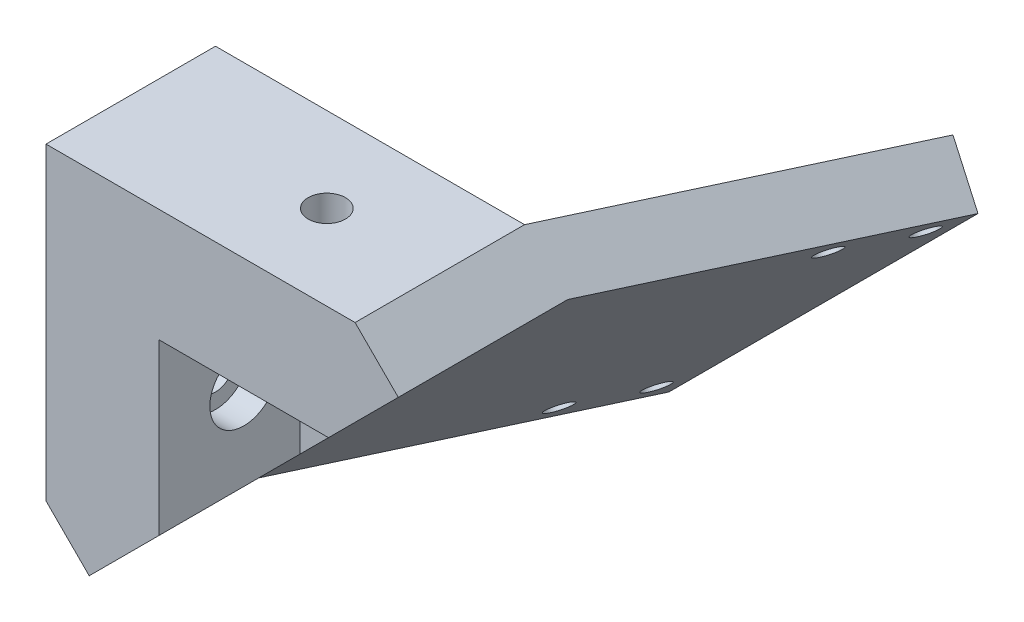
from build123d import *

# Parameters (mm, degrees)
EXTRUDE_1_DEPTH      = 15
EXTRUDE_2_DEPTH      = 49.497475
EXTRUDE_2_DEPTH_BACK = 49.497475
CUT_EXTRUDE_3_DEPTH  = 113
SKETCH_8_R           = 3.3
CUT_EXTRUDE_4_DEPTH  = 113
CUT_EXTRUDE_START    = -15
SKETCH_9_R           = 6
CUT_EXTRUDE_5_DEPTH  = 113
CUT_EXTRUDE_6_DEPTH  = 25
SKETCH_11_R          = 2.2
CUT_EXTRUDE_7_DEPTH  = 30


with BuildPart() as part:
    # 草图1 → 凸台-拉伸1 (new, symmetric)
    with BuildSketch(Plane.XY):
        Polygon((0, 0), (70, 0), (0, -70), align=None)
    extrude(amount=EXTRUDE_1_DEPTH, both=True)

    # 草图5 → 凸台-拉伸2 (add, two sides: drawn at the far end of the back side and taken through both)
    with BuildSketch(Plane(origin=(0, 0, 0), x_dir=(0.7071067811865476, -0.7071067811865476, 0), z_dir=(-0.7071067811865476, -0.7071067811865476, 0)).offset(-EXTRUDE_2_DEPTH_BACK)):
        Polygon((65.854033042, -76.043506833), (49.497474683, -15), (38.68197258, -15), (55.763032203, -78.747382359), align=None)
    extrude(amount=EXTRUDE_2_DEPTH + EXTRUDE_2_DEPTH_BACK)

    # 草图7 → 切除-拉伸3 (cut)
    with BuildSketch(Plane.XY.offset(15)):
        Polygon((70, 0), (54.704570242, 0), (62.352285121, -7.647714879), align=None)
        Polygon((62.352285121, 7.647714879), (54.704570242, 0), (70, 0), align=None)
        Polygon((70, 0), (62.352285121, -7.647714879), (73.918118454, -19.213548212), (81.565833333, -11.565833333), align=None)
        Polygon((19.213548212, -73.918118454), (7.647714879, -62.352285121), (0, -70), (11.565833333, -81.565833333), align=None)
        Polygon((0, -70), (7.647714879, -62.352285121), (0, -54.704570242), align=None)
        Polygon((0, -70), (0, -54.704570242), (-7.647714879, -62.352285121), align=None)
    extrude(amount=-CUT_EXTRUDE_3_DEPTH, mode=Mode.SUBTRACT)

    # 草图8 → 切除-拉伸4 (cut)
    with BuildSketch(Plane(origin=(0, 0, 0), x_dir=(1, 0, 0), z_dir=(0, 1, 0))):
        with Locations(Location((34.704570242, 0, 0), (0, 0, 270))):
            Circle(SKETCH_8_R)
    cut_extrude_4 = extrude(amount=-CUT_EXTRUDE_4_DEPTH, mode=Mode.SUBTRACT)

    # 草图9 → 切除-拉伸5 (cut)
    with BuildSketch(Plane(origin=(0, 0, 0), x_dir=(1, 0, 0), z_dir=(0, 1, 0)).offset(CUT_EXTRUDE_START)):
        with Locations(Location((34.704570242, 0, 0), (0, 0, 270))):
            Circle(SKETCH_9_R)
    cut_extrude_5 = extrude(amount=-CUT_EXTRUDE_5_DEPTH, mode=Mode.SUBTRACT)

    # 草图10 → 切除-拉伸6 (cut)
    with BuildSketch(Plane.XY.offset(15)):
        Polygon((20, -20), (20, -50), (47.352285121, -22.647714879), (50, -20), align=None)
    extrude(amount=-CUT_EXTRUDE_6_DEPTH, mode=Mode.SUBTRACT)

    # 镜向2: 切除-拉伸4, 切除-拉伸5 across plane
    add(cut_extrude_4.mirror(Plane(origin=(0, 0, 0), x_dir=(0, 0, 1), z_dir=(-0.7071067811865476, -0.7071067811865476, 0))), mode=Mode.SUBTRACT)
    add(cut_extrude_5.mirror(Plane(origin=(0, 0, 0), x_dir=(0, 0, 1), z_dir=(-0.7071067811865476, -0.7071067811865476, 0))), mode=Mode.SUBTRACT)

    # 草图11 → 切除-拉伸7 (cut)
    with BuildSketch(Plane(origin=(30.003794137, -30.003794137, 11.369559199), x_dir=(0.18301270189221028, -0.18301270189221025, -0.9659258262890718), z_dir=(0.6830127018922219, -0.6830127018922217, 0.25881904510250797))):
        with Locations(Location((70.49666512, 33.68197258, 0), (0, 0, 90))):
            Circle(SKETCH_11_R)
        with Locations(Location((85.49666512, 33.68197258, 0), (0, 0, 90))):
            Circle(SKETCH_11_R)
        with Locations(Location((85.49666512, -33.68197258, 0), (0, 0, 90))):
            Circle(SKETCH_11_R)
        with Locations(Location((70.49666512, -33.68197258, 0), (0, 0, 90))):
            Circle(SKETCH_11_R)
    extrude(amount=-CUT_EXTRUDE_7_DEPTH, mode=Mode.SUBTRACT)


solid = part.part
